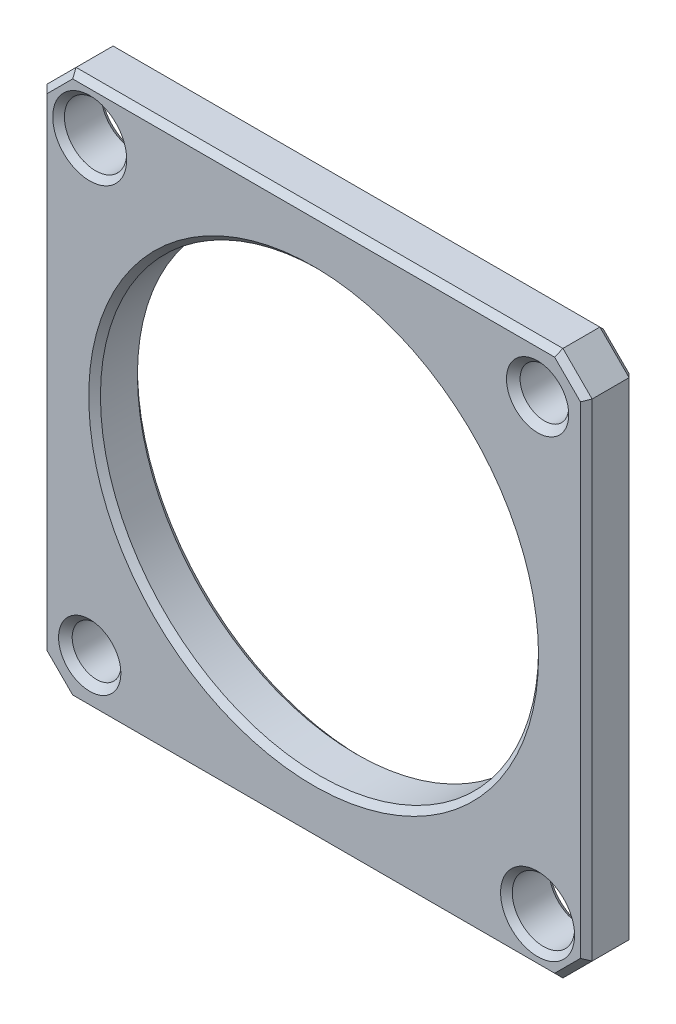
from build123d import *

# Parameters (mm, degrees)
SKETCH1_R                  = 11.25
BOSS_EXTRUDE1_DEPTH        = 2.5
SKETCH2_R                  = 1.6
CUT_EXTRUDE1_DEPTH         = 2.5
M3_TAPPED_HOLE1_AT_2_COUNT = 2
M3_TAPPED_HOLE1_AT_2_PITCH = 32.526911935
CHAMFER1_SIZE              = 0.3


with BuildPart() as part:
    # Sketch1 → Boss-Extrude1 (new body)
    with BuildSketch(Plane.XY):
        Polygon((-14, -12.5), (-12.5, -14), (12.5, -14), (14, -12.5), (14, 12.5), (12.5, 14), (-12.5, 14), (-14, 12.5), align=None)
        Circle(SKETCH1_R, mode=Mode.SUBTRACT)
    extrude(amount=BOSS_EXTRUDE1_DEPTH)

    # Sketch2 → Cut-Extrude1 (cut)
    with BuildSketch(Plane.XY.offset(2.5)):
        with Locations((-11.5, 11.5)):
            Circle(SKETCH2_R)
        with Locations((11.5, -11.5)):
            Circle(SKETCH2_R)
    extrude(amount=-CUT_EXTRUDE1_DEPTH, mode=Mode.SUBTRACT)

    # Sketch4 → M3 Tapped Hole1 (revolve, cut)
    with BuildSketch(Plane(origin=(-11.5, -11.5, 2.5), x_dir=(0, -1, 0), z_dir=(1, 0, 0))):
        Polygon((0, 0), (0, 2.5), (1.6, 2.5), (1.25, 2.15), (1.25, 0.35), (1.6, 0), align=None)
    m3_tapped_hole1 = revolve(axis=Axis((-11.5, -11.5, 8.85), (0, 0, -1)), mode=Mode.SUBTRACT)

    # M3 Tapped Hole1 at 2: M3 Tapped Hole1 ×2
    with Locations(*[Vector(0.7071067811865476, 0.7071067811865476, 0) * (i * M3_TAPPED_HOLE1_AT_2_PITCH) for i in range(1, M3_TAPPED_HOLE1_AT_2_COUNT)]):
        add(m3_tapped_hole1, mode=Mode.SUBTRACT)

    # Chamfer1
    chamfer1_edges = [part.edges().sort_by_distance(p)[0] for p in [
        (13.25, -13.25, 0),
        (0, -14, 0),
        (-13.25, -13.25, 0),
        (-14, 0, 0),
        (0, -14, 2.5),
        (13.25, -13.25, 2.5),
        (14, 0, 2.5),
        (-11.25, 0, 0),
        (-11.25, 0, 2.5),
        (13.25, 13.25, 2.5),
        (0, 14, 2.5),
        (-13.1, 11.5, 0),
        (-13.1, 11.5, 2.5),
        (-13.25, 13.25, 2.5),
        (9.9, -11.5, 0),
        (9.9, -11.5, 2.5),
        (-14, 0, 2.5),
        (-13.25, 13.25, 0),
        (-13.25, -13.25, 2.5),
        (0, 14, 0),
        (13.25, 13.25, 0),
        (14, 0, 0),
    ]]
    chamfer(chamfer1_edges, length=CHAMFER1_SIZE)


solid = part.part
